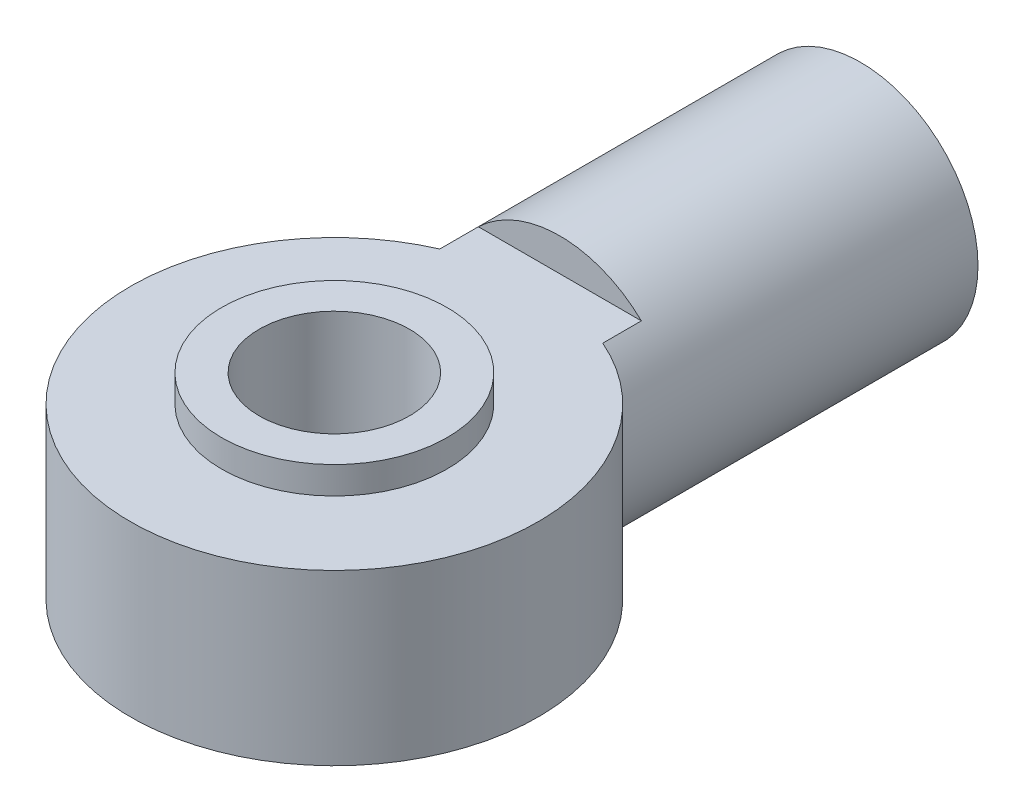
from build123d import *
from build123d.topology import SkipClean

# Parameters (mm, degrees)
SKETCH_1_R             = 6.25
EXTRUDE_1_DEPTH        = 28
SKETCH_2_R             = 10.85
EXTRUDE_2_DEPTH        = 4.5
CUT_EXTRUDE_START      = -12
CUT_EXTRUDE_1_DEPTH    = 12
SKETCH_4_R             = 4
CUT_EXTRUDE_2_DEPTH    = 42.744550687
HOLE_WIZARD_M8_1_D     = 6.8
HOLE_WIZARD_M8_1_DEPTH = 12
HOLE_WIZARD_M8_1_TIP   = 2.042926105
SKETCH_8_R             = 6
SKETCH_8_R_2           = 4
EXTRUDE_3_DEPTH        = 5.95


with BuildPart() as part:
    # 草图1 → 凸台-拉伸1 (new body)
    with BuildSketch(Plane.XY):
        Circle(SKETCH_1_R)
    extrude(amount=EXTRUDE_1_DEPTH)

    # 草图2 → 凸台-拉伸2 (add, symmetric)
    with BuildSketch(Plane(origin=(0, 0, 0), x_dir=(1, 0, 0), z_dir=(0, 1, 0))):
        with Locations((0, -28)):
            Circle(SKETCH_2_R)
    extrude(amount=EXTRUDE_2_DEPTH, both=True)

    # 草图3 → 切除-拉伸1 (cut)
    with BuildSketch(Plane.XY.offset(28).offset(CUT_EXTRUDE_START)):
        with BuildLine():
            Line((4.337337893, -4.5), (-4.337337893, -4.5))
            ThreePointArc((-4.337337893, -4.5), (0, -6.25), (4.337337893, -4.5))
        make_face()
        with BuildLine():
            Line((-4.337337893, 4.5), (4.337337893, 4.5))
            ThreePointArc((4.337337893, 4.5), (0, 6.25), (-4.337337893, 4.5))
        make_face()
    extrude(amount=CUT_EXTRUDE_1_DEPTH, mode=Mode.SUBTRACT)

    # 草图4 → 切除-拉伸2 (cut, through all)
    with BuildSketch(Plane.XZ.offset(4.5)):
        with Locations(Location((0, 28, 0), (0, 0, 270))):
            Circle(SKETCH_4_R)
    extrude(amount=-CUT_EXTRUDE_2_DEPTH, mode=Mode.SUBTRACT)

    # M8 螺纹孔1
    with Locations(Plane(origin=(0, 0, 0), x_dir=(-1, 0, 0), z_dir=(0, 0, -1))):
        with Locations((0, 0)):
            Hole(HOLE_WIZARD_M8_1_D / 2, depth=HOLE_WIZARD_M8_1_DEPTH)
            with Locations((0, 0, -(HOLE_WIZARD_M8_1_DEPTH + HOLE_WIZARD_M8_1_TIP / 2))):  # 118° drill point
                Cone(0, HOLE_WIZARD_M8_1_D / 2, HOLE_WIZARD_M8_1_TIP, mode=Mode.SUBTRACT)

    # 草图8 → 凸台-拉伸3 (add, symmetric)
    with SkipClean():  # the faces are left unmerged after this step: merging them gives an invalid solid
        with BuildSketch(Plane(origin=(0, 0, 0), x_dir=(1, 0, 0), z_dir=(0, 1, 0))):
            with Locations(Location((0, -28, 0), (0, 0, 270))):
                Circle(SKETCH_8_R)
            with Locations(Location((0, -28, 0), (0, 0, 270))):
                Circle(SKETCH_8_R_2, mode=Mode.SUBTRACT)
        extrude(amount=EXTRUDE_3_DEPTH, both=True)


solid = part.part
